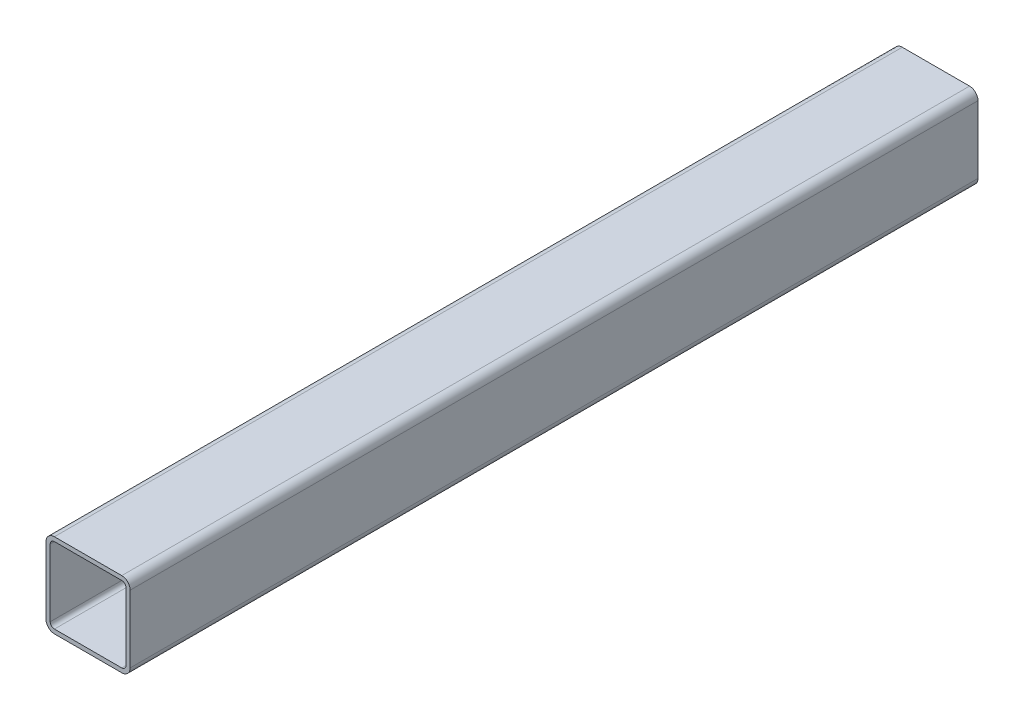
from build123d import *

# Parameters (mm, degrees)
SKETCH1_W           = 40
SKETCH1_H           = 40
SKETCH1_W_2         = 36
SKETCH1_H_2         = 36
BOSS_EXTRUDE1_DEPTH = 403
FILLET1_R           = 2
FILLET2_R           = 4


with BuildPart() as part:
    # Sketch1 → Boss-Extrude1 (new body)
    with BuildSketch(Plane.XY):
        Rectangle(SKETCH1_W, SKETCH1_H)
        Rectangle(SKETCH1_W_2, SKETCH1_H_2, mode=Mode.SUBTRACT)
    extrude(amount=BOSS_EXTRUDE1_DEPTH)

    # Fillet1
    fillet1_edges = [part.edges().sort_by_distance(p)[0] for p in [
        (18, -18, 201.5),
        (18, 18, 201.5),
        (-18, 18, 201.5),
        (-18, -18, 201.5),
    ]]
    fillet(fillet1_edges, radius=FILLET1_R)

    # Fillet2
    fillet2_edges = [part.edges().sort_by_distance(p)[0] for p in [
        (20, -20, 201.5),
        (-20, -20, 201.5),
        (-20, 20, 201.5),
        (20, 20, 201.5),
    ]]
    fillet(fillet2_edges, radius=FILLET2_R)


solid = part.part
